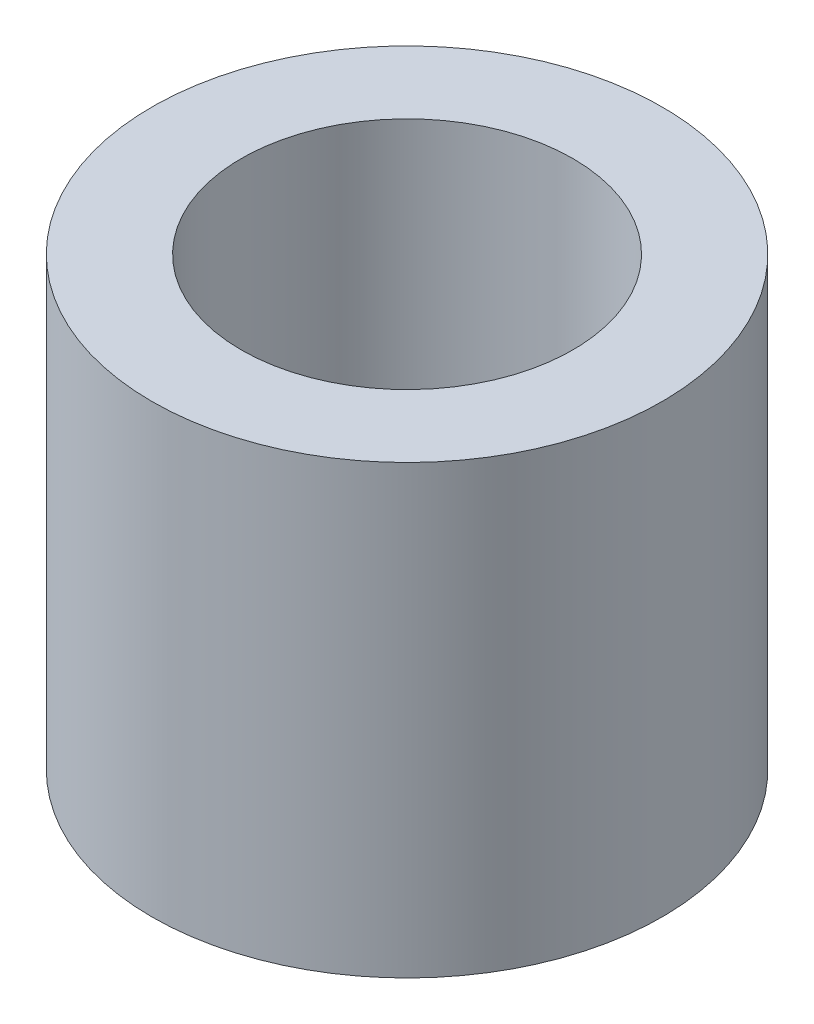
from build123d import *

# Parameters (mm, degrees)
SKETCH1_R           = 4
SKETCH1_R_2         = 2.6
BOSS_EXTRUDE1_DEPTH = 7


with BuildPart() as part:
    # Sketch1 → Boss-Extrude1 (new body)
    with BuildSketch(Plane(origin=(0, 0, 0), x_dir=(1, 0, 0), z_dir=(0, 1, 0))):
        with Locations(Location((0, 0, 0), (0, 0, 270))):
            Circle(SKETCH1_R)
        with Locations(Location((0, 0, 0), (0, 0, 270))):
            Circle(SKETCH1_R_2, mode=Mode.SUBTRACT)
    extrude(amount=BOSS_EXTRUDE1_DEPTH)


solid = part.part
